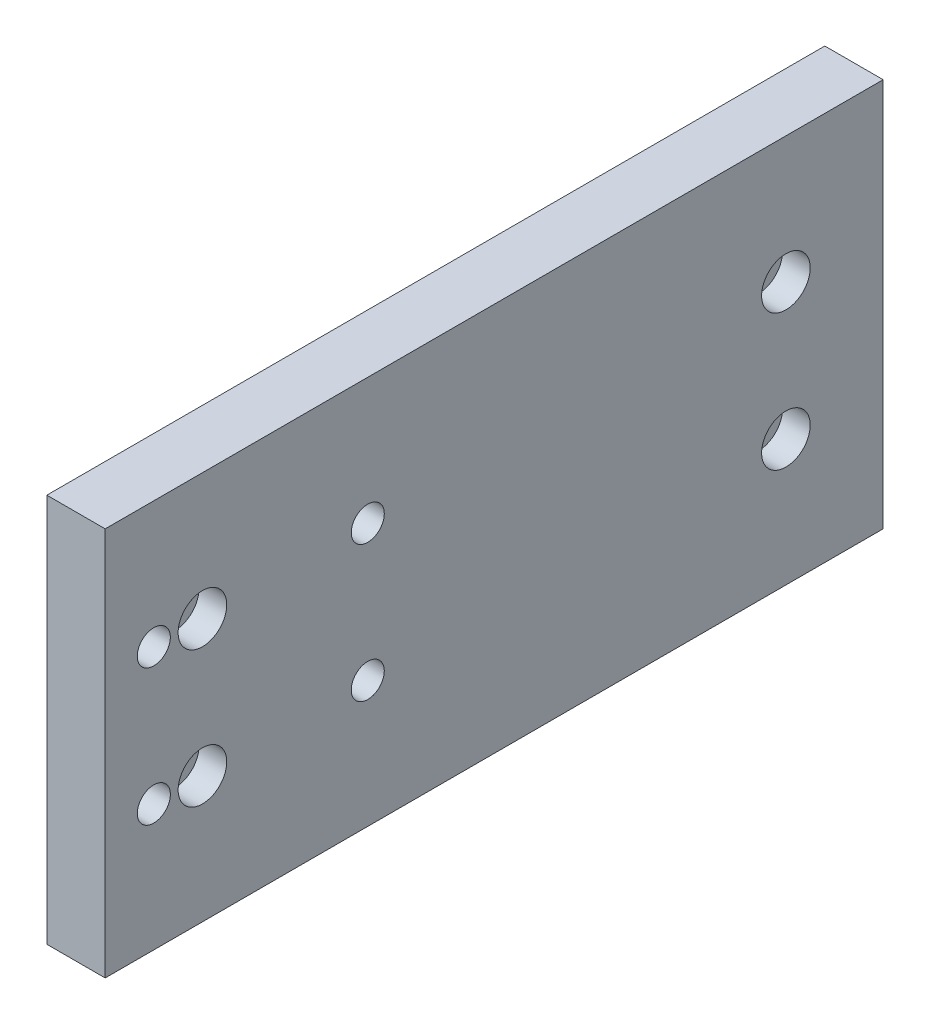
from build123d import *

# Parameters (mm, degrees)
SKETCH_1_W                = 160
SKETCH_1_H                = 80
EXTRUDE_1_DEPTH           = 12
HOLE_WIZARD_M8_1_D        = 6.8
HOLE_WIZARD_1_D           = 5.5
HOLE_WIZARD_1_CBORE_D     = 10
HOLE_WIZARD_1_CBORE_DEPTH = 5.7


with BuildPart() as part:
    # 草图1 → 凸台-拉伸1 (new body)
    with BuildSketch(Plane(origin=(0, 0, 0), x_dir=(0, 0, -1), z_dir=(1, 0, 0))):
        Rectangle(SKETCH_1_W, SKETCH_1_H)
    extrude(amount=EXTRUDE_1_DEPTH)

    # M8 螺纹孔1 (through all)
    with Locations(Plane(origin=(12, 0, 0), x_dir=(0, 0, -1), z_dir=(1, 0, 0))):
        with Locations((-70, 14), (-70, -14), (-26, 14), (-26, -14)):
            Hole(HOLE_WIZARD_M8_1_D / 2)

    # 打孔尺寸(%根据)内六角圆柱头螺钉的类型1 (through all)
    with Locations(Plane(origin=(12, 0, 0), x_dir=(0, 0, -1), z_dir=(1, 0, 0))):
        with Locations((-60, 14), (-60, -14), (60, 14), (60, -14)):
            CounterBoreHole(HOLE_WIZARD_1_D / 2, HOLE_WIZARD_1_CBORE_D / 2, HOLE_WIZARD_1_CBORE_DEPTH)


solid = part.part
